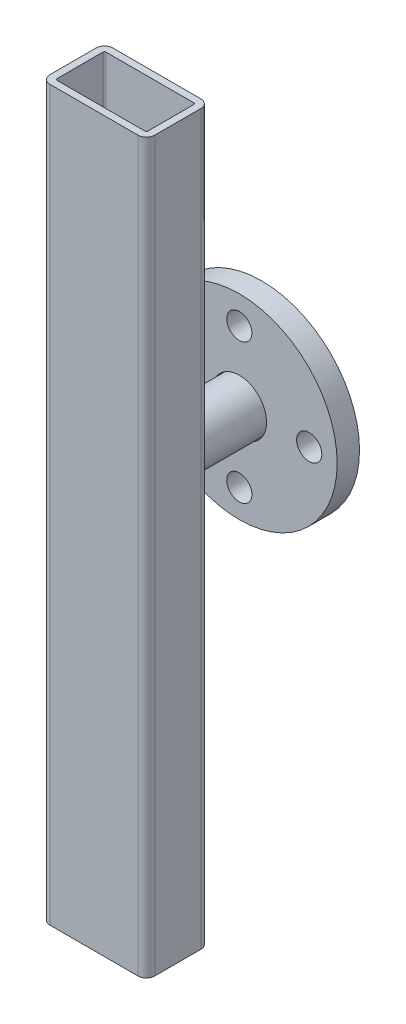
SolidWorks part; units mm, degrees
ref_plane "Front" through (0, 0, 0) normal (0, 0, 1) x (1, 0, 0)
ref_plane "Top" through (0, 0, 0) normal (0, 1, 0) x (1, 0, 0)
ref_plane "Right" through (0, 0, 0) normal (1, 0, 0) x (0, 0, -1)
sketch "草图1" plane through (0, 0, 0) normal (0, 1, 0) x (1, 0, 0)
  line L0 (-44, -2.2781) -> (19, -2.2781)
  line L1 (-44, -7.2781) -> (19, -7.2781)
  line L2 (-50, -1.2781) -> (-50, 31.7219)
  line L3 (-44, 37.7219) -> (19, 37.7219)
  line L4 (25, -1.2781) -> (25, 31.7219)
  line L5 (20, -1.2781) -> (20, 31.7219)
  line L6 (-44, 32.7219) -> (19, 32.7219)
  line L11 (-45, -1.2781) -> (-45, 31.7219)
  arc A0 (-44, -7.2781) -> (-50, -1.2781) centre (-44, -1.2781) cw
  arc A1 (19, -7.2781) -> (25, -1.2781) centre (19, -1.2781) ccw
  arc A2 (19, 37.7219) -> (25, 31.7219) centre (19, 31.7219) cw
  arc A3 (-50, 31.7219) -> (-44, 37.7219) centre (-44, 31.7219) cw
  arc A4 (19, -2.2781) -> (20, -1.2781) centre (19, -1.2781) ccw
  arc A5 (19, 32.7219) -> (20, 31.7219) centre (19, 31.7219) cw
  arc A6 (-45, 31.7219) -> (-44, 32.7219) centre (-44, 31.7219) cw
  arc A7 (-44, -2.2781) -> (-45, -1.2781) centre (-44, -1.2781) cw
  point P9 (25, -7.2781)
  point P12 (25, 37.7219)
  point P15 (-50, 37.7219)
  dimension "D3" = 6
  dimension "D1" = 75
  dimension "D2" = 45
  dimension "D4" = 5
extrude "凸台-拉伸1" add sketch "草图1" along normal blind 521
sketch "草图2" plane through (0, 0, -37.7219) normal (0, 0, -1) x (-1, 0, 0)
  line L0 (-25, 521) -> (-25, 0) construction
  line L1 (-19, 0) -> (44, 0) construction
  circle A0 centre (12.5, 285) radius 19
  dimension "D1" = 38
  dimension "D2" = 37.5
  dimension "D3" = 285
extrude "凸台-拉伸2" add sketch "草图2" along normal blind 75
sketch "草图3" plane through (0, 0, -112.7219) normal (0, 0, -1) x (-1, 0, 0)
  circle A0 centre (12.5, 285) radius 70
  circle A1 centre (12.5, 285) radius 50 construction
  circle A2 centre (12.5, 335) radius 9
  circle A3 centre (62.5, 285) radius 9
  circle A4 centre (12.5, 235) radius 9
  circle A5 centre (-37.5, 285) radius 9
  point P15 (12.5, 285)
  dimension "D1" = 140
  dimension "D2" = 100
  dimension "D3" = 18
  dimension "D4" = 4
extrude "凸台-拉伸3" add sketch "草图3" against normal blind 16
sketch "草图4" plane through (0, 0, -112.7219) normal (0, 0, -1) x (-1, 0, 0)
  circle A0 centre (12.5, 285) radius 39
  dimension "D1" = 78
extrude "凸台-拉伸4" add sketch "草图4" along normal blind 2
sketch "草图5" plane through (0, 0, -114.7219) normal (0, 0, -1) x (-1, 0, 0)
  circle A0 centre (12.5, 285) radius 19.5
  circle A1 centre (12.5, 285) radius 19
  dimension "D1" = 39
  dimension "D2" = 38
extrude "切除-拉伸1" cut sketch "草图5" against normal up to surface (77 mm away) up to face at (6.5, 285, -37.7219)
